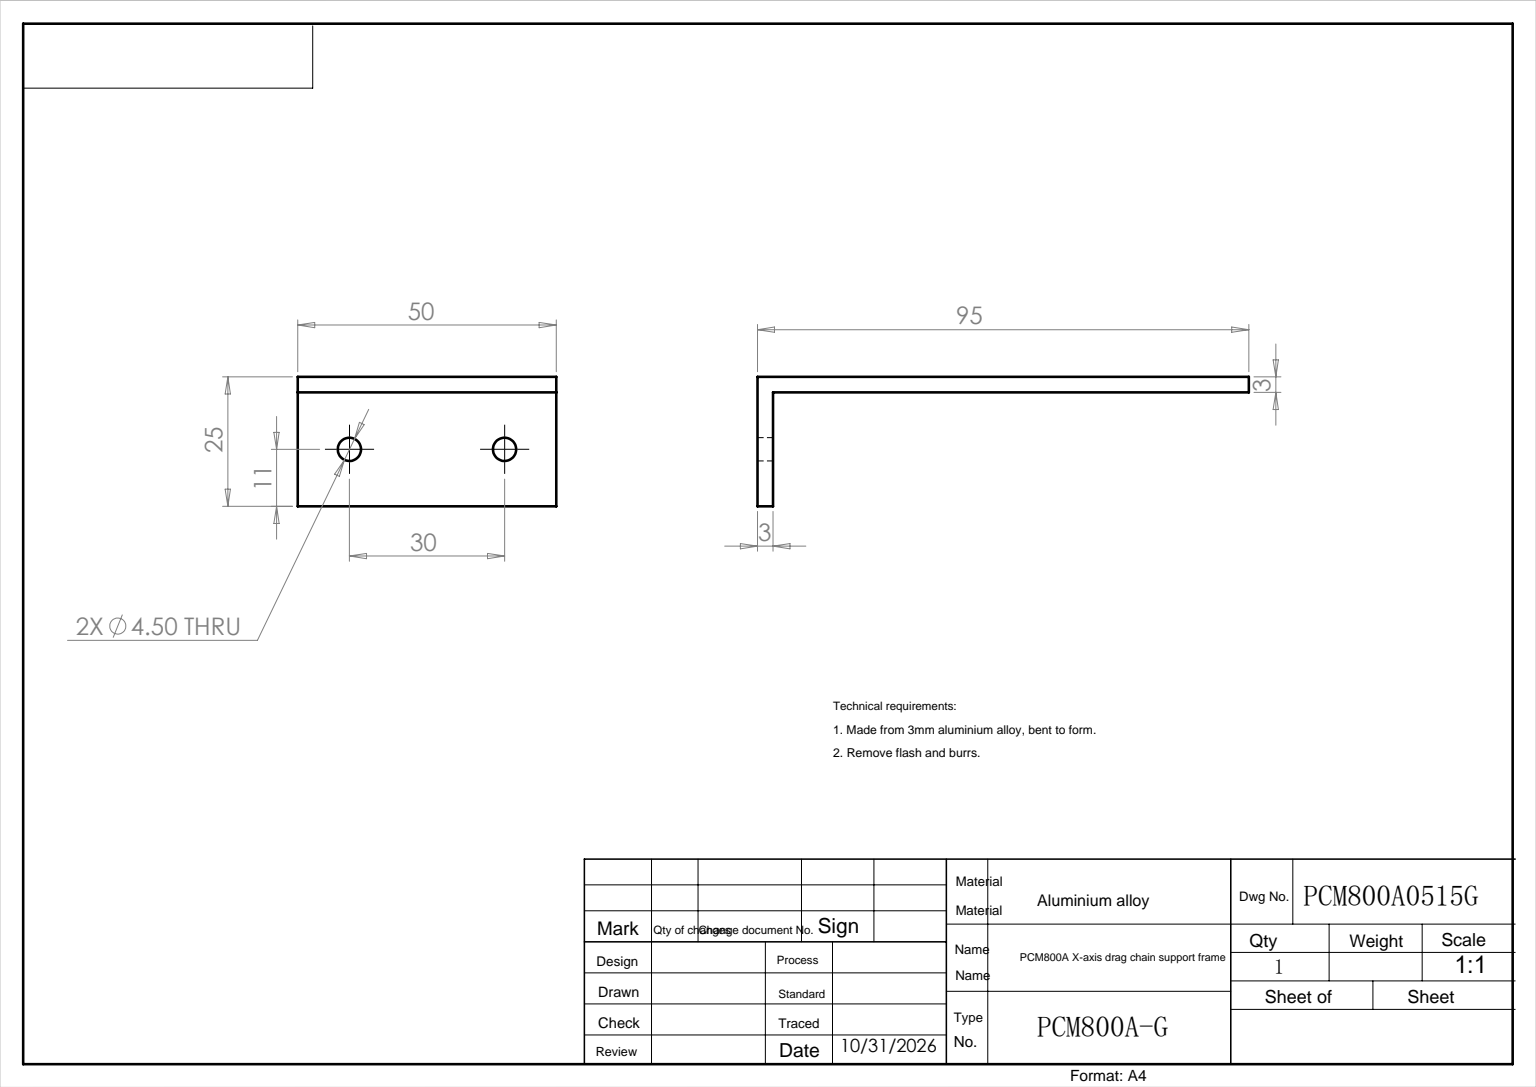
from build123d import *

# Parameters (mm, degrees)
EXTRUDE_1_DEPTH     = 50
SKETCH_2_R          = 2.25
CUT_EXTRUDE_1_DEPTH = 10


with BuildPart() as part:
    # 草图1 → 拉伸-薄壁1 (new body)
    with BuildSketch(Plane.XY):
        Polygon((0, 0), (0, 25), (95, 25), (95, 22), (3, 22), (3, 0), align=None)
    extrude(amount=EXTRUDE_1_DEPTH)

    # 草图2 → 切除-拉伸1 (cut)
    with BuildSketch(Plane(origin=(3, 0, 0), x_dir=(0, 0, -1), z_dir=(1, 0, 0))):
        with Locations((-40, 11)):
            Circle(SKETCH_2_R)
        with Locations(Location((-10, 11, 0), (0, 0, 180))):
            Circle(SKETCH_2_R)
    extrude(amount=-CUT_EXTRUDE_1_DEPTH, mode=Mode.SUBTRACT)


solid = part.part
